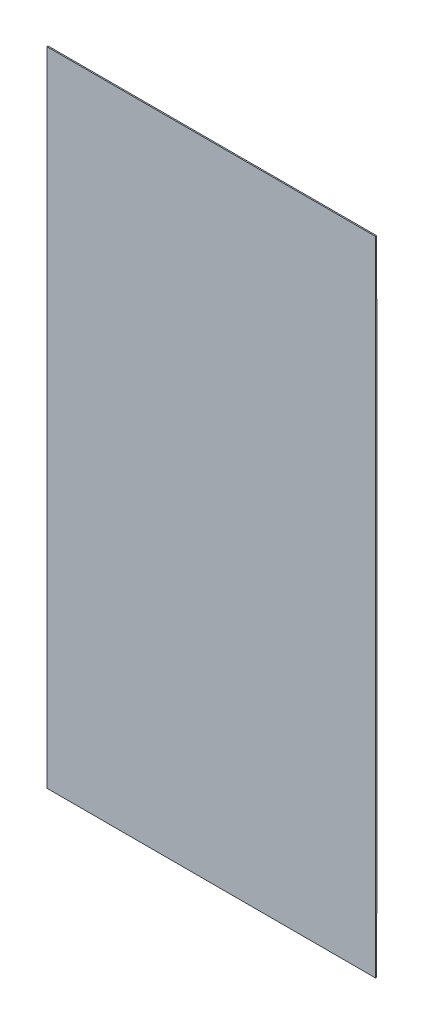
SolidWorks part; units mm, degrees
ref_plane "前视" through (0, 0, 0) normal (0, 0, 1) x (1, 0, 0)
ref_plane "上视" through (0, 0, 0) normal (0, 1, 0) x (1, 0, 0)
ref_plane "右视" through (0, 0, 0) normal (1, 0, 0) x (0, 0, -1)
sketch "草图1" plane through (0, 0, 0) normal (0, 0, 1) x (1, 0, 0)
  line L1 (0, 0) -> (1100, 0)
  line L2 (0, 0) -> (0, -2150)
  line L3 (0, -2150) -> (1100, -2150)
  line L4 (1100, 0) -> (1100, -2150)
  dimension "D1" = 1100
  dimension "D2" = 2150
extrude "凸台-拉伸1" add sketch "草图1" along normal blind 4
sketch "草图2" plane through (0, 0, 0) normal (0, 0, -1) x (-1, 0, 0)
  line L0 (-1100, -2150) -> (-1100, 0) construction
  line L1 (-1100, -1965) -> (0, -1965)
  line L2 (-1100, -1965) -> (-1100, -185)
  line L3 (-1100, -185) -> (0, -185)
  line L4 (0, -1965) -> (0, -185)
  line L5 (0, 0) -> (0, -2150) construction
  line L6 (0, -2150) -> (-1100, -2150) construction
  line L7 (-1100, 0) -> (0, 0) construction
  dimension "D1" = 185
  dimension "D2" = 185
extrude "凸台-拉伸2" add sketch "草图2" along normal blind 1
